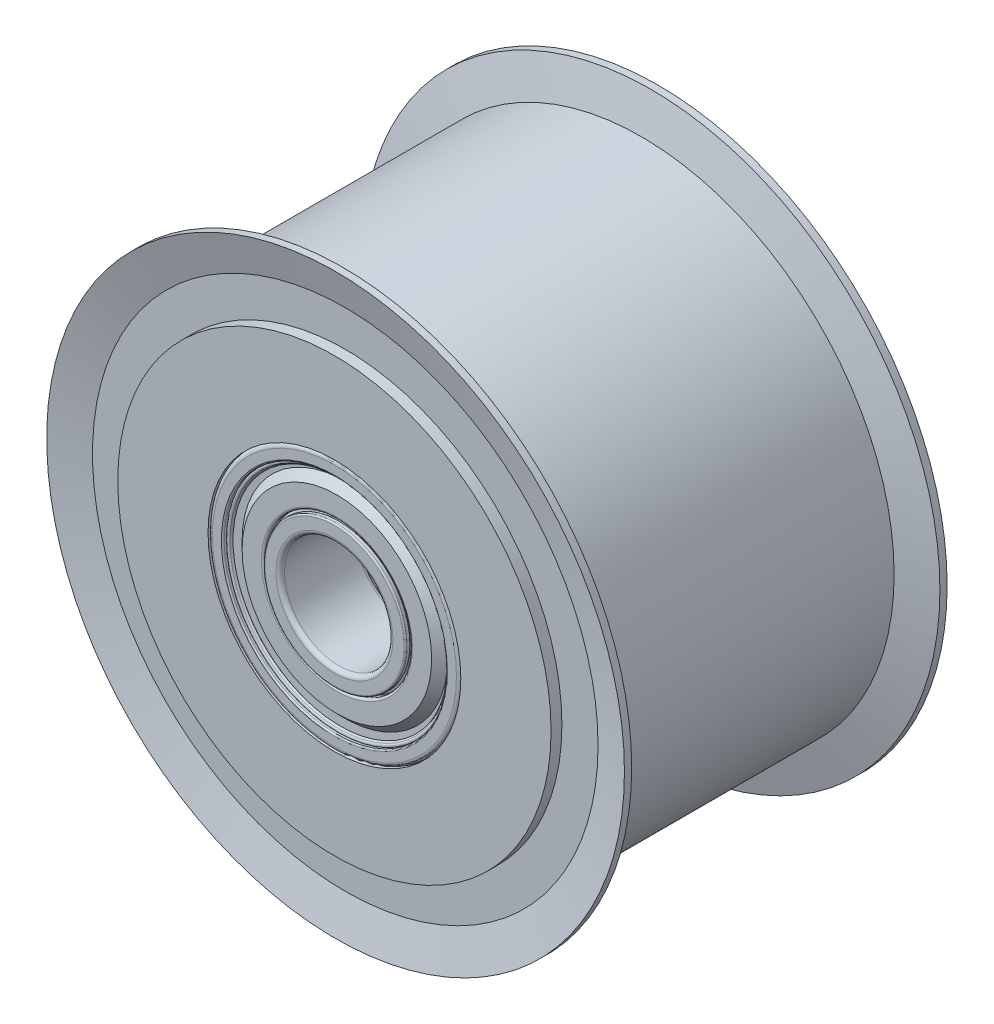
from build123d import *


with BuildPart() as part:
    # 草图1 → 旋转1 (revolve)
    with BuildSketch(Plane(origin=(0, 0, 0), x_dir=(0, 0, -1), z_dir=(1, 0, 0)), mode=Mode.PRIVATE) as revolve_1_sk:
        Polygon((0, 17.5), (11, 17.5), (11, 12.75), (34, 12.75), (34, 17.5), (45, 17.5), (45, 30), (43.5, 30), (43.5, 35), (44.839745962, 40), (43.839745962, 40), (42.5, 35), (2.5, 35), (1.160254038, 40), (0.160254038, 40), (1.5, 35), (1.5, 30), (0, 30), align=None)
    revolve(revolve_1_sk.sketch.rotate(Axis((0, 0, -45), (0, 0, 1)), 270), axis=Axis((0, 0, -45), (0, 0, 1)))

    # 草图2 → 旋转2 (revolve)
    with BuildSketch(Plane(origin=(0, 0, 0), x_dir=(0, 0, -1), z_dir=(1, 0, 0)), mode=Mode.PRIVATE) as revolve_2_sk:
        with BuildLine():
            Line((0.2, 15.45), (0.5, 15.45))
            ThreePointArc((0.5, 15.45), (0.45029759, 15.226027188), (0.573393587, 15.032425726))
            Line((0.573393587, 15.032425726), (0.819, 14.86))
            Line((0.819, 14.86), (0.991, 15.105))
            Line((0.991, 15.105), (0.746, 15.278))
            Line((0.746, 15.278), (1.028401172, 15.680571884))
            ThreePointArc((1.028401172, 15.680571884), (1.24881307, 15.757515702), (1.391995431, 15.573123274))
            Line((1.391995431, 15.573123274), (1.442, 14.224))
            Line((1.442, 14.224), (0.342, 13.124))
            Line((0.342, 13.124), (0.342, 10.45))
            ThreePointArc((0.342, 10.45), (0.429867966, 10.237867966), (0.642, 10.15))
            Line((0.642, 10.15), (1.162, 10.15))
            Line((1.162, 10.15), (1.162, 10.45))
            Line((1.162, 10.45), (0.642, 10.45))
            Line((0.642, 10.45), (0.642, 13))
            Line((0.642, 13), (1.742, 14.1))
            Line((1.742, 14.1), (1.742, 14.45))
            Line((1.742, 14.45), (2.994, 14.45))
            ThreePointArc((2.994, 14.45), (2.324618686, 12.5), (2.994, 10.55))
            Line((2.994, 10.55), (1.945085653, 10.55))
            ThreePointArc((1.945085653, 10.55), (1.830383283, 10.513839453), (1.757157918, 10.418433662))
            Line((1.757157918, 10.418433662), (1.434206231, 9.531566338))
            ThreePointArc((1.434206231, 9.531566338), (1.360980866, 9.436160547), (1.246278495, 9.4))
            Line((1.246278495, 9.4), (1.070837627, 9.4))
            ThreePointArc((1.070837627, 9.4), (0.986311342, 9.41873967), (0.917625005, 9.471446929))
            Line((0.917625005, 9.471446929), (0.6, 9.85))
            Line((0.6, 9.85), (0.2, 9.85))
            ThreePointArc((0.2, 9.85), (0.058578644, 9.791421356), (0, 9.65))
            Line((0, 9.65), (0, 8.1))
            ThreePointArc((0, 8.1), (0.175735931, 7.675735931), (0.6, 7.5))
            Line((0.6, 7.5), (10.4, 7.5))
            ThreePointArc((10.4, 7.5), (10.824264069, 7.675735931), (11, 8.1))
            Line((11, 8.1), (11, 9.65))
            ThreePointArc((11, 9.65), (10.941421356, 9.791421356), (10.8, 9.85))
            Line((10.8, 9.85), (10.4, 9.85))
            Line((10.4, 9.85), (10.082374995, 9.471446929))
            ThreePointArc((10.082374995, 9.471446929), (10.013688658, 9.41873967), (9.929162373, 9.4))
            Line((9.929162373, 9.4), (9.753721505, 9.4))
            ThreePointArc((9.753721505, 9.4), (9.639019134, 9.436160547), (9.565793769, 9.531566338))
            Line((9.565793769, 9.531566338), (9.242842082, 10.418433662))
            ThreePointArc((9.242842082, 10.418433662), (9.169616717, 10.513839453), (9.054914347, 10.55))
            Line((9.054914347, 10.55), (8.006, 10.55))
            ThreePointArc((8.006, 10.55), (8.675381314, 12.5), (8.006, 14.45))
            Line((8.006, 14.45), (9.258, 14.45))
            Line((9.258, 14.45), (9.258, 14.1))
            Line((9.258, 14.1), (10.358, 13))
            Line((10.358, 13), (10.358, 10.45))
            Line((10.358, 10.45), (9.838, 10.45))
            Line((9.838, 10.45), (9.838, 10.15))
            Line((9.838, 10.15), (10.358, 10.15))
            ThreePointArc((10.358, 10.15), (10.570132034, 10.237867966), (10.658, 10.45))
            Line((10.658, 10.45), (10.658, 13.124))
            Line((10.658, 13.124), (9.558, 14.224))
            Line((9.558, 14.224), (9.608004569, 15.573123274))
            ThreePointArc((9.608004569, 15.573123274), (9.75118693, 15.757515702), (9.971598828, 15.680571884))
            Line((9.971598828, 15.680571884), (10.254, 15.278))
            Line((10.254, 15.278), (10.009, 15.105))
            Line((10.009, 15.105), (10.181, 14.86))
            Line((10.181, 14.86), (10.426606413, 15.032425726))
            ThreePointArc((10.426606413, 15.032425726), (10.54970241, 15.226027188), (10.5, 15.45))
            Line((10.5, 15.45), (10.8, 15.45))
            ThreePointArc((10.8, 15.45), (10.941421356, 15.508578644), (11, 15.65))
            Line((11, 15.65), (11, 16.9))
            ThreePointArc((11, 16.9), (10.824264069, 17.324264069), (10.4, 17.5))
            Line((10.4, 17.5), (0.6, 17.5))
            ThreePointArc((0.6, 17.5), (0.175735931, 17.324264069), (0, 16.9))
            Line((0, 16.9), (0, 15.65))
            ThreePointArc((0, 15.65), (0.058578644, 15.508578644), (0.2, 15.45))
        make_face()
    revolve(revolve_2_sk.sketch.rotate(Axis((0, 0, -50), (0, 0, 1)), 270), axis=Axis((0, 0, -50), (0, 0, 1)))

    # 草图3 → 旋转3 (revolve)
    with BuildSketch(Plane(origin=(0, 0, 0), x_dir=(0, 0, -1), z_dir=(1, 0, 0)), mode=Mode.PRIVATE) as revolve_3_sk:
        with BuildLine():
            Line((34.2, 15.45), (34.5, 15.45))
            ThreePointArc((34.5, 15.45), (34.45029759, 15.226027188), (34.573393587, 15.032425726))
            Line((34.573393587, 15.032425726), (34.819, 14.86))
            Line((34.819, 14.86), (34.991, 15.105))
            Line((34.991, 15.105), (34.746, 15.278))
            Line((34.746, 15.278), (35.028401172, 15.680571884))
            ThreePointArc((35.028401172, 15.680571884), (35.24881307, 15.757515702), (35.391995431, 15.573123274))
            Line((35.391995431, 15.573123274), (35.442, 14.224))
            Line((35.442, 14.224), (34.342, 13.124))
            Line((34.342, 13.124), (34.342, 10.45))
            ThreePointArc((34.342, 10.45), (34.429867966, 10.237867966), (34.642, 10.15))
            Line((34.642, 10.15), (35.162, 10.15))
            Line((35.162, 10.15), (35.162, 10.45))
            Line((35.162, 10.45), (34.642, 10.45))
            Line((34.642, 10.45), (34.642, 13))
            Line((34.642, 13), (35.742, 14.1))
            Line((35.742, 14.1), (35.742, 14.45))
            Line((35.742, 14.45), (36.994, 14.45))
            ThreePointArc((36.994, 14.45), (36.324618686, 12.5), (36.994, 10.55))
            Line((36.994, 10.55), (35.945085653, 10.55))
            ThreePointArc((35.945085653, 10.55), (35.830383283, 10.513839453), (35.757157918, 10.418433662))
            Line((35.757157918, 10.418433662), (35.434206231, 9.531566338))
            ThreePointArc((35.434206231, 9.531566338), (35.360980866, 9.436160547), (35.246278495, 9.4))
            Line((35.246278495, 9.4), (35.070837627, 9.4))
            ThreePointArc((35.070837627, 9.4), (34.986311342, 9.41873967), (34.917625005, 9.471446929))
            Line((34.917625005, 9.471446929), (34.6, 9.85))
            Line((34.6, 9.85), (34.2, 9.85))
            ThreePointArc((34.2, 9.85), (34.058578644, 9.791421356), (34, 9.65))
            Line((34, 9.65), (34, 8.1))
            ThreePointArc((34, 8.1), (34.175735931, 7.675735931), (34.6, 7.5))
            Line((34.6, 7.5), (44.4, 7.5))
            ThreePointArc((44.4, 7.5), (44.824264069, 7.675735931), (45, 8.1))
            Line((45, 8.1), (45, 9.65))
            ThreePointArc((45, 9.65), (44.941421356, 9.791421356), (44.8, 9.85))
            Line((44.8, 9.85), (44.4, 9.85))
            Line((44.4, 9.85), (44.082374995, 9.471446929))
            ThreePointArc((44.082374995, 9.471446929), (44.013688658, 9.41873967), (43.929162373, 9.4))
            Line((43.929162373, 9.4), (43.753721505, 9.4))
            ThreePointArc((43.753721505, 9.4), (43.639019134, 9.436160547), (43.565793769, 9.531566338))
            Line((43.565793769, 9.531566338), (43.242842082, 10.418433662))
            ThreePointArc((43.242842082, 10.418433662), (43.169616717, 10.513839453), (43.054914347, 10.55))
            Line((43.054914347, 10.55), (42.006, 10.55))
            ThreePointArc((42.006, 10.55), (42.675381314, 12.5), (42.006, 14.45))
            Line((42.006, 14.45), (43.258, 14.45))
            Line((43.258, 14.45), (43.258, 14.1))
            Line((43.258, 14.1), (44.358, 13))
            Line((44.358, 13), (44.358, 10.45))
            Line((44.358, 10.45), (43.838, 10.45))
            Line((43.838, 10.45), (43.838, 10.15))
            Line((43.838, 10.15), (44.358, 10.15))
            ThreePointArc((44.358, 10.15), (44.570132034, 10.237867966), (44.658, 10.45))
            Line((44.658, 10.45), (44.658, 13.124))
            Line((44.658, 13.124), (43.558, 14.224))
            Line((43.558, 14.224), (43.608004569, 15.573123274))
            ThreePointArc((43.608004569, 15.573123274), (43.75118693, 15.757515702), (43.971598828, 15.680571884))
            Line((43.971598828, 15.680571884), (44.254, 15.278))
            Line((44.254, 15.278), (44.009, 15.105))
            Line((44.009, 15.105), (44.181, 14.86))
            Line((44.181, 14.86), (44.426606413, 15.032425726))
            ThreePointArc((44.426606413, 15.032425726), (44.54970241, 15.226027188), (44.5, 15.45))
            Line((44.5, 15.45), (44.8, 15.45))
            ThreePointArc((44.8, 15.45), (44.941421356, 15.508578644), (45, 15.65))
            Line((45, 15.65), (45, 16.9))
            ThreePointArc((45, 16.9), (44.824264069, 17.324264069), (44.4, 17.5))
            Line((44.4, 17.5), (34.6, 17.5))
            ThreePointArc((34.6, 17.5), (34.175735931, 17.324264069), (34, 16.9))
            Line((34, 16.9), (34, 15.65))
            ThreePointArc((34, 15.65), (34.058578644, 15.508578644), (34.2, 15.45))
        make_face()
    revolve(revolve_3_sk.sketch.rotate(Axis((0, 0, -50), (0, 0, 1)), 270), axis=Axis((0, 0, -50), (0, 0, 1)))


solid = part.part
